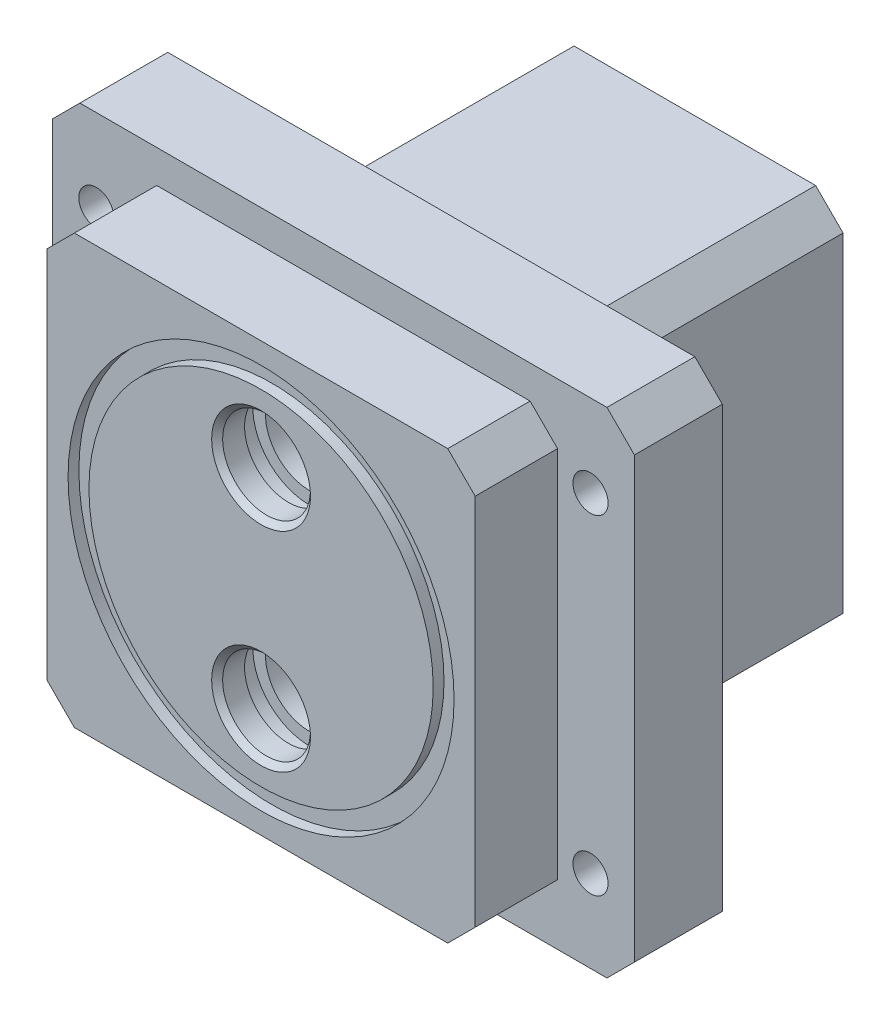
from build123d import *

# Parameters (mm, degrees)
SKETCH1_W             = 54
SKETCH1_H             = 70
BOSS_EXTRUDE1_DEPTH   = 48
SKETCH2_W             = 106
SKETCH2_H             = 90
BOSS_EXTRUDE2_DEPTH   = 16
SKETCH3_W             = 78
SKETCH3_H             = 78
BOSS_EXTRUDE3_DEPTH   = 15
CHAMFER1_SIZE         = 5
SKETCH4_R             = 35.15
SKETCH4_R_2           = 31.35
CUT_EXTRUDE1_DEPTH    = 1.97
HOLE1_D               = 16
HOLE2_D               = 22
HOLE2_DEPTH           = 63
CHAMFER2_SIZE         = 1
M5_TAPPED_HOLE1_D     = 4.2
M5_TAPPED_HOLE1_DEPTH = 10
M5_TAPPED_HOLE1_TIP   = 1.2618073
HOLE3_D               = 6.4
HOLE3_CBORE_D         = 11
HOLE3_CBORE_DEPTH     = 9
SKETCH16_R            = 10.3
CUT_EXTRUDE2_DEPTH    = 3.8


with BuildPart() as part:
    # Sketch1 → Boss-Extrude1 (new body)
    with BuildSketch(Plane.XY):
        Rectangle(SKETCH1_W, SKETCH1_H)
    extrude(amount=BOSS_EXTRUDE1_DEPTH)

    # Sketch2 → Boss-Extrude2 (add)
    with BuildSketch(Plane.XY.offset(48)):
        Rectangle(SKETCH2_W, SKETCH2_H)
    extrude(amount=BOSS_EXTRUDE2_DEPTH)

    # Sketch3 → Boss-Extrude3 (add)
    with BuildSketch(Plane.XY.offset(64)):
        Rectangle(SKETCH3_W, SKETCH3_H)
    extrude(amount=BOSS_EXTRUDE3_DEPTH)

    # Chamfer1
    chamfer1_edges = [part.edges().sort_by_distance(p)[0] for p in [
        (-53, 45, 56),
        (-53, -45, 56),
        (53, -45, 56),
        (53, 45, 56),
        (-39, 39, 71.5),
        (-39, -39, 71.5),
        (39, -39, 71.5),
        (39, 39, 71.5),
        (27, -35, 24),
        (-27, -35, 24),
        (-27, 35, 24),
        (27, 35, 24),
    ]]
    chamfer(chamfer1_edges, length=CHAMFER1_SIZE)

    # Sketch4 → Cut-Extrude1 (cut)
    with BuildSketch(Plane.XY.offset(79)):
        Circle(SKETCH4_R)
        Circle(SKETCH4_R_2, mode=Mode.SUBTRACT)
    extrude(amount=-CUT_EXTRUDE1_DEPTH, mode=Mode.SUBTRACT)

    # Hole1 (through all)
    with Locations(Plane.XY.offset(79)):
        with Locations((0, -19), (0, 19)):
            Hole(HOLE1_D / 2)

    # Hole2
    with Locations(Plane(origin=(0, 0, 0), x_dir=(-1, 0, 0), z_dir=(0, 0, -1))):
        with Locations((0, 19), (0, -19)):
            Hole(HOLE2_D / 2, depth=HOLE2_DEPTH)

    # Chamfer2
    chamfer2_edges = [part.edges().sort_by_distance(p)[0] for p in [
        (8, 19, 79),
        (8, -19, 79),
        (-11, -19, 0),
        (-11, 19, 0),
    ]]
    chamfer(chamfer2_edges, length=CHAMFER2_SIZE)

    # M5 Tapped Hole1
    with Locations(Plane(origin=(0, 0, 0), x_dir=(-1, 0, 0), z_dir=(0, 0, -1))):
        with Locations((20, -19), (20, 19), (-20, 19), (-20, -19)):
            Hole(M5_TAPPED_HOLE1_D / 2, depth=M5_TAPPED_HOLE1_DEPTH)
            with Locations((0, 0, -(M5_TAPPED_HOLE1_DEPTH + M5_TAPPED_HOLE1_TIP / 2))):  # 118° drill point
                Cone(0, M5_TAPPED_HOLE1_D / 2, M5_TAPPED_HOLE1_TIP, mode=Mode.SUBTRACT)

    # Hole3 (through all)
    with Locations(Plane(origin=(0, 0, 48), x_dir=(-1, 0, 0), z_dir=(0, 0, -1))):
        with Locations((45, -30), (45, 30), (-45, 30), (-45, -30)):
            CounterBoreHole(HOLE3_D / 2, HOLE3_CBORE_D / 2, HOLE3_CBORE_DEPTH)

    # Sketch16 → Cut-Extrude2 (cut)
    with BuildSketch(Plane.XY.offset(74)):
        with Locations((0, 19)):
            Circle(SKETCH16_R)
        with Locations((0, -19)):
            Circle(SKETCH16_R)
    extrude(amount=-CUT_EXTRUDE2_DEPTH, mode=Mode.SUBTRACT)


solid = part.part
